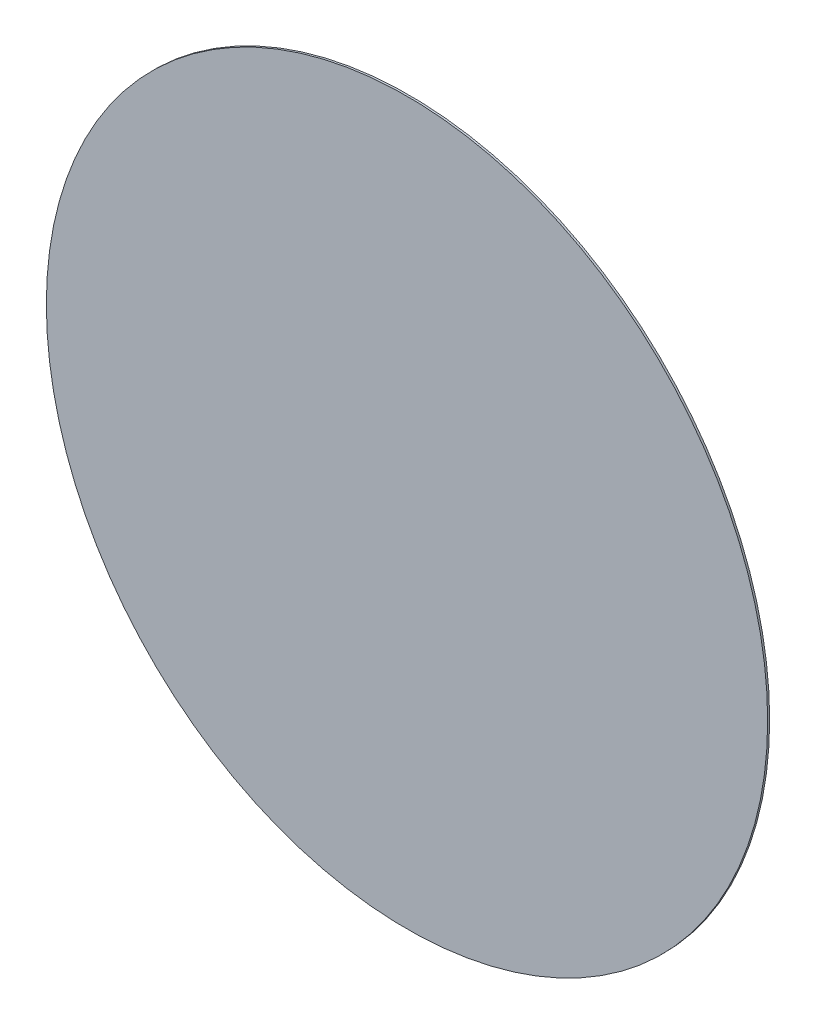
SolidWorks part; units mm, degrees
material "ABS"
ref_plane "前视" through (0, 0, 0) normal (0, 0, 1) x (1, 0, 0)
ref_plane "上视" through (0, 0, 0) normal (0, 1, 0) x (1, 0, 0)
ref_plane "右视" through (0, 0, 0) normal (1, 0, 0) x (0, 0, -1)
sketch "草图1" plane through (0, 0, 0) normal (0, 0, 1) x (1, 0, 0)
  circle A0 centre (0, 0) radius 54
extrude "凸台-拉伸1" add sketch "草图1" along normal blind 0.3
